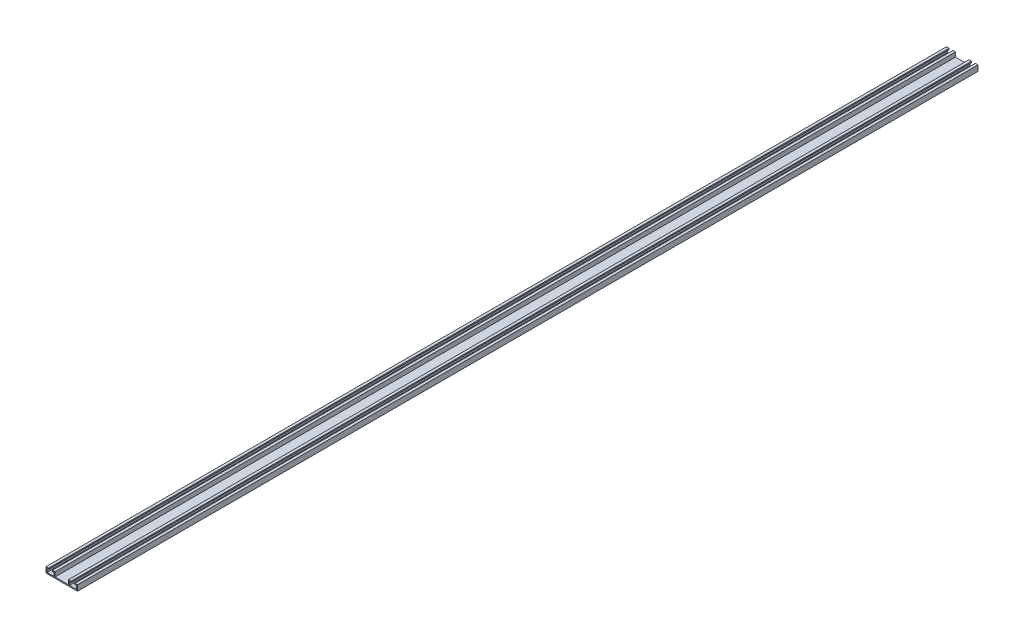
SolidWorks part; units mm, degrees
ref_plane "前视基准面" through (0, 0, 0) normal (0, 0, 1) x (1, 0, 0)
ref_plane "上视基准面" through (0, 0, 0) normal (0, 1, 0) x (1, 0, 0)
ref_plane "右视基准面" through (0, 0, 0) normal (1, 0, 0) x (0, 0, -1)
sketch "草图1" plane through (0, 0, 0) normal (0, 0, 1) x (1, 0, 0)
  line L0 (0, 0) -> (8, 0)
  line L1 (8, 0) -> (8, 5)
  line L2 (8, 5) -> (5.65, 5)
  line L3 (0, 0) -> (0, 5)
  line L4 (0, 5) -> (2.35, 5)
  line L5 (4, 0) -> (4, 6.7213) construction
  dimension "D1" = 3.3
  dimension "D2" = 8
  dimension "D3" = 5
extrude "拉伸-薄壁1" add sketch "草图1" along normal blind 800 thin thin type one direction wall 1
sketch "草图2" plane through (0, 0, 800) normal (0, 0, 1) x (1, 0, 0)
  line L0 (0, 0) -> (-6, 0)
  line L1 (8, 5) -> (8, 0) construction
  dimension "D1" = 14
extrude "拉伸-薄壁2" add sketch "草图2" against normal up to surface (800 mm away) thin
mirror "镜向1" about plane through (-6, 0, -6.0828) normal (1, 0, 0) of bodies 107
sketch "草图5" plane through (0, 1, 0) normal (0, 1, 0) x (1, 0, 0)
  line L0 (-19, 0) -> (-13, 0) construction
  line L1 (-20, -800) -> (-20, 0) construction
  line L2 (0, -400) -> (-66.3884, -400) construction
  line L3 (0, 0) -> (0, -800) construction
  point P0 (-16, -10)
  point P14 (-16, -790)
  dimension "D1" = 10
  dimension "D2" = 4
hole_wizard "M3 间隙孔1" positions "草图5" profile "草图4" hole size "M3" standard "GB"
sketch "草图4" plane through (-16, 1, 10) normal (1, 0, 0) x (0, 0, 1)
  line L0 (0, 0) -> (0, 1)
  line L1 (0, 1) -> (1.7, 1)
  line L2 (1.7, 1) -> (1.7, 0)
  line L5 (1.7, 0) -> (0, 0)
  line L11 (0, -6.35) -> (0, 107.95) construction
  dimension "通孔孔直径" = 3.4
  dimension "通孔孔深度" = 1
